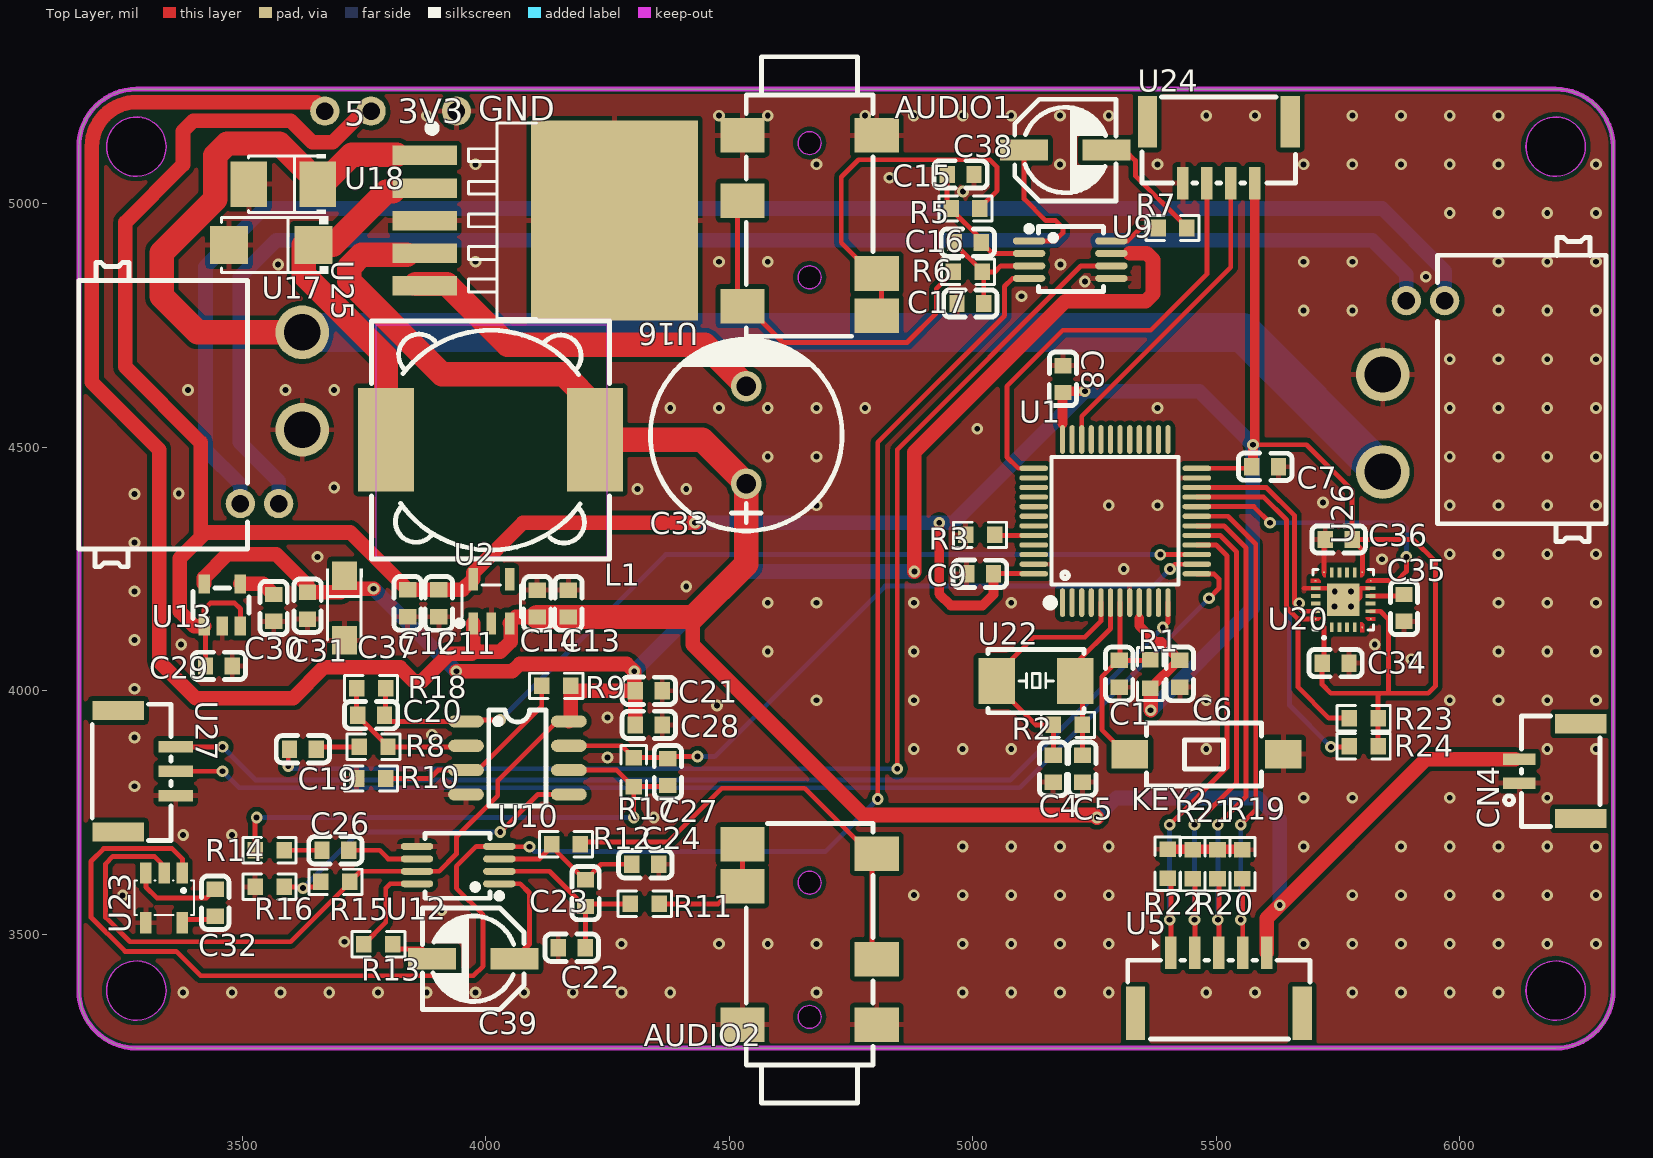
[diagram p0: Top Layer view]
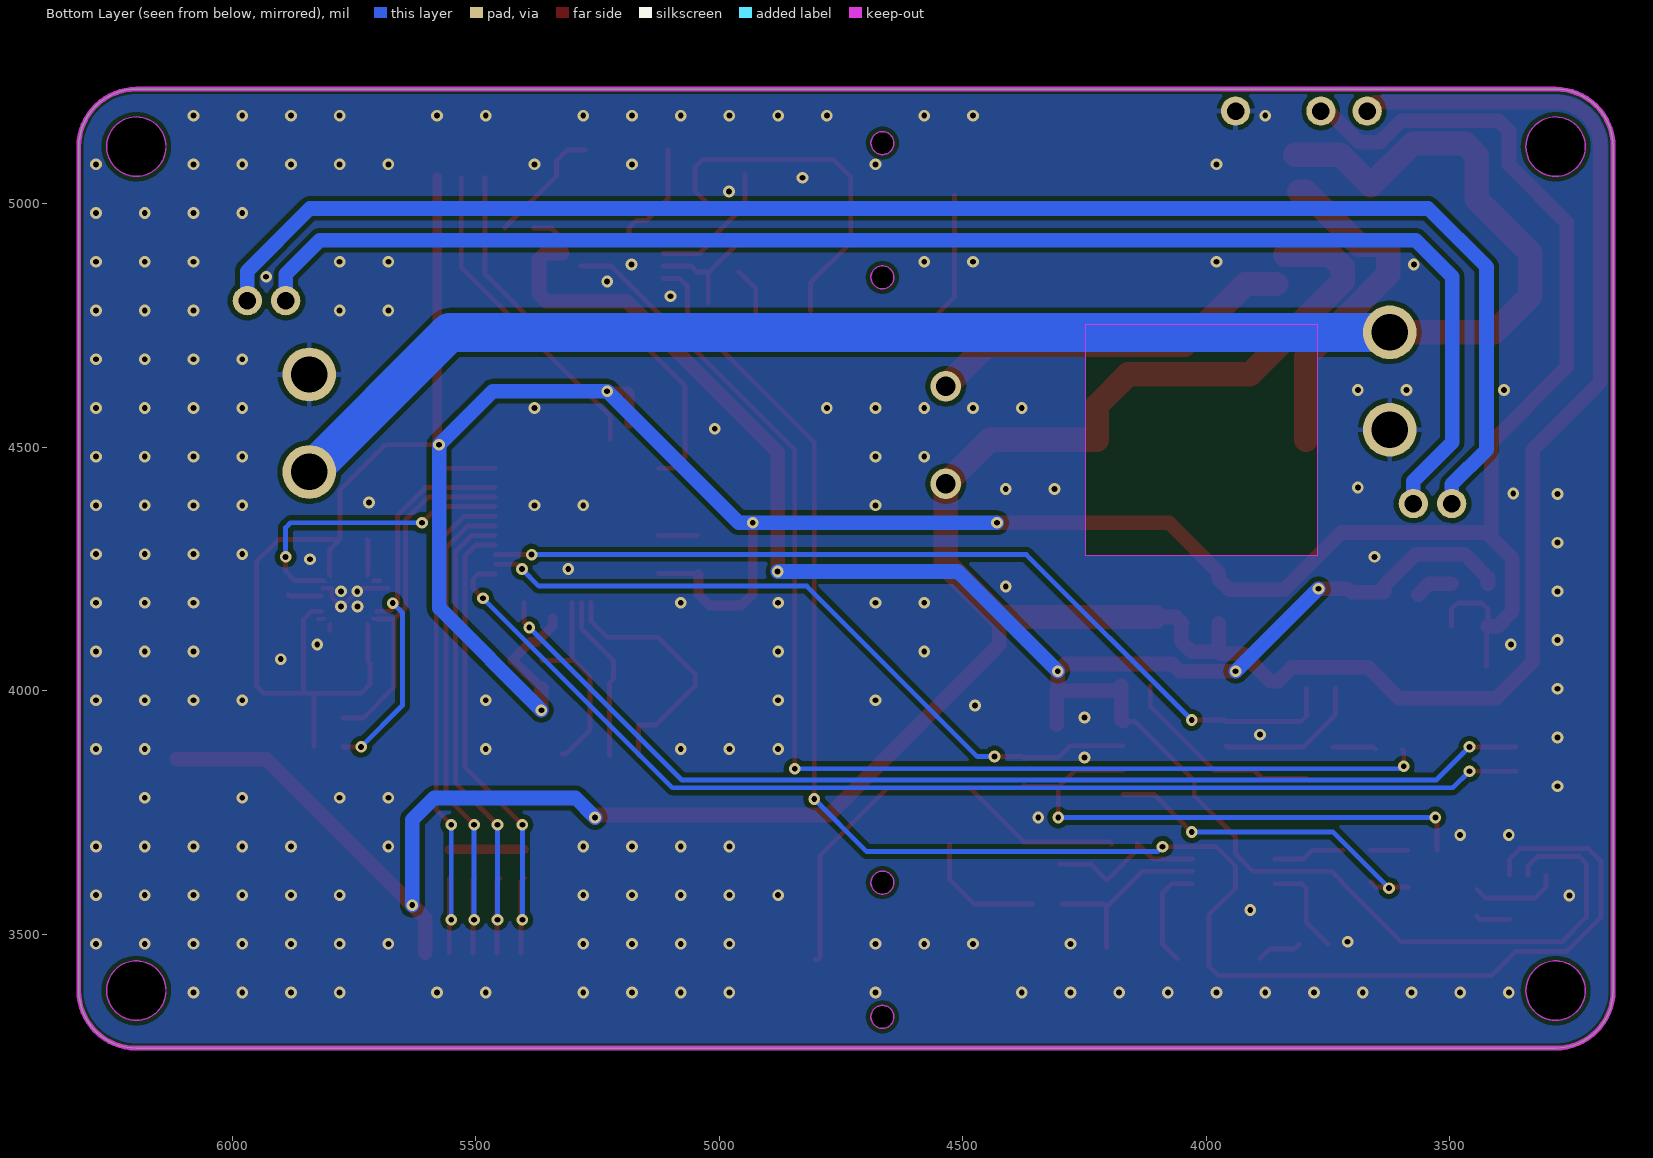
[diagram p1: Bottom Layer view, seen from below]
# Altium PCB MISC61403.pcbdoc
Units mil, origin at the board's own origin, x right, y up, seen from the top; angles counter-clockwise.
Board outline 3149.61 x 1968.5 mil, 2 copper layers (Top Layer, Bottom Layer), stack 62.206 mil thick; 79 components, 75 nets, 287 pads, 243 vias.

## Layer stack, top to bottom
Top Solder Mask Layer: solder mask 0.394, Dk 3.3
Top Layer: signal copper 1.379
Dielectric1: surface 59.449, FR4, Dk 4.5
Bottom Layer: signal copper 1.378
Bottom Solder Mask Layer: solder mask 0.394, Dk 3.3

## Board outline
3283.11,5235 ccw(c3283.11,5116.89) 3165,5116.89 3165,3384.61 ccw(c3283.11,3384.61) 3283.11,3266.5 6196.5,3266.5 ccw(c6196.5,3384.61) 6314.61,3384.61 6314.61,5116.89 ccw(c6196.5,5116.89) 6196.5,5235
cut-out: 3344.13,5116.89 cw(c3283.11,5116.89) 3222.09,5116.89 cw(c3283.11,5116.89)
cut-out: 3344.13,3384.61 cw(c3283.11,3384.61) 3222.09,3384.61 cw(c3283.11,3384.61)
cut-out: 6257.52,3384.61 cw(c6196.5,3384.61) 6135.47,3384.61 cw(c6196.5,3384.61)
cut-out: 6257.52,5116.89 cw(c6196.5,5116.89) 6135.47,5116.89 cw(c6196.5,5116.89)

## Design rules (kind name [scope] priority, off if disabled: settings)
BoardOutlineClearance Plane_innerPlane_1 [All] p2 off: genericclearance=6 ignorepadtopadclearanceinfootprint=FALSE except(0: Arc-SplitContinuation Track-SplitContinuation SMDPad-SplitContinuation THPad-SplitContinuation Via-SplitContinuation Fill-SplitContinuation Region-SplitContinuation Poly-SplitContinuation Text-SplitContinuation Hole-SplitContinuation; 6: Arc-CutoutEdge Track-CutoutEdge SMDPad-CutoutEdge THPad-CutoutEdge Via-CutoutEdge Fill-CutoutEdge Region-CutoutEdge Text-CutoutEdge Hole-CutoutEdge; 10: Poly-OutlineEdge Poly-CutoutEdge; 11.8: Arc-OutlineEdge Track-OutlineEdge SMDPad-OutlineEdge THPad-OutlineEdge Via-OutlineEdge Fill-OutlineEdge Region-OutlineEdge Text-OutlineEdge Hole-OutlineEdge)
BoardOutlineClearance Copper_copperRegion_1 [All] p4 off: genericclearance=6 ignorepadtopadclearanceinfootprint=FALSE except(0: Arc-SplitContinuation Track-SplitContinuation SMDPad-SplitContinuation THPad-SplitContinuation Via-SplitContinuation Fill-SplitContinuation Region-SplitContinuation Poly-SplitContinuation Text-SplitContinuation Hole-SplitContinuation; 6: Arc-CutoutEdge Track-CutoutEdge SMDPad-CutoutEdge THPad-CutoutEdge Via-CutoutEdge Fill-CutoutEdge Region-CutoutEdge Text-CutoutEdge Hole-CutoutEdge; 10: Poly-OutlineEdge Poly-CutoutEdge; 11.8: Arc-OutlineEdge Track-OutlineEdge SMDPad-OutlineEdge THPad-OutlineEdge Via-OutlineEdge Fill-OutlineEdge Region-OutlineEdge Text-OutlineEdge Hole-OutlineEdge)
BoardOutlineClearance safeClearance_1 [All] p6: genericclearance=6 ignorepadtopadclearanceinfootprint=FALSE except(0: Arc-SplitContinuation Track-SplitContinuation SMDPad-SplitContinuation THPad-SplitContinuation Via-SplitContinuation Fill-SplitContinuation Region-SplitContinuation Poly-SplitContinuation Text-SplitContinuation Hole-SplitContinuation; 6: Arc-CutoutEdge Track-CutoutEdge SMDPad-CutoutEdge THPad-CutoutEdge Via-CutoutEdge Fill-CutoutEdge Region-CutoutEdge Text-CutoutEdge Hole-CutoutEdge; 10: Poly-OutlineEdge Poly-CutoutEdge; 11.8: Arc-OutlineEdge Track-OutlineEdge SMDPad-OutlineEdge THPad-OutlineEdge Via-OutlineEdge Fill-OutlineEdge Region-OutlineEdge Text-OutlineEdge Hole-OutlineEdge)
Clearance Plane_innerPlane [All] p1 off: gap=6 ignorepadtopadclearanceinfootprint=FALSE except(10: Poly-Track Poly-SMDPad Poly-THPad Poly-Via Poly-Fill Poly-Region Poly-Poly Poly-Arc Poly-Text Poly-Hole)
Clearance Copper_copperRegion [All] p3 off: gap=6 ignorepadtopadclearanceinfootprint=FALSE except(10: Poly-Track Poly-SMDPad Poly-THPad Poly-Via Poly-Fill Poly-Region Poly-Poly Poly-Arc Poly-Text Poly-Hole)
Clearance safeClearance [All] p5: gap=6 ignorepadtopadclearanceinfootprint=FALSE except(10: Poly-Track Poly-SMDPad Poly-THPad Poly-Via Poly-Fill Poly-Region Poly-Poly Poly-Arc Poly-Text Poly-Hole)
DiffPairsRouting differentialPair [All] p1: maxlimit=6 minlimit=6 mostfreqgap=6 toplayer_minwidth=5 toplayer_prefwidth=10 toplayer_maxwidth=100 toplayer_mingap=6 toplayer_prefgap=6 toplayer_maxgap=6 bottomlayer_minwidth=5 bottomlayer_prefwidth=10 bottomlayer_maxwidth=100 bottomlayer_mingap=6 bottomlayer_prefgap=6 bottomlayer_maxgap=6 maxuncoupledlength=10
HoleToHoleClearance otherClearance [All] p1: gap=11.8 allowstackedmicrovias=TRUE
Length netLength [All] p1: minlimit=0 maxlimit=0
PasteMaskExpansion pasteMaskExpansion [All] p1: expansion=0
PlaneConnect innerPlane [All] p1: planeconnectstyle=Relief reliefexpansion=20 reliefentries=4 reliefconductorwidth=10 reliefairgap=10
PolygonConnect copperRegion [All] p1: connectstyle=Relief reliefconductorwidth=10 reliefentries=4 polygonreliefangle="90 Angle" airgapwidth=10 via.connectstyle=Relief via.reliefconductorwidth=10 via.reliefentries=4 via.polygonreliefangle="90 Angle" via.airgapwidth=10
RoutingVias viaSize [All] p1: holewidth=12.01 width=24.02 viastyle="Through Hole" minholewidth=11.81 minwidth=19.68 maxholewidth=236.22 maxwidth=393.7
SolderMaskExpansion solderMaskExpansion [IsVia] p1: expansion=-1000 istentingtop=TRUE
SolderMaskExpansion solderMaskExpansion [All] p2: expansion=2 istentingtop=FALSE
Width trackWidth [All] p1: maxlimit=100 minlimit=5 preferedwidth=10

## Components (designator, comment, footprint, x,y, rotation, side; value= is the part's Value field where it differs from the comment)
AUDIO1 "PJ-3420-A-SMT" AUDIO-SMD_PJ-3420-A-SMT_C319102 4665,4955 r270 top
AUDIO2 "PJ-3420-A-SMT" AUDIO-SMD_PJ-3420-A-SMT_C319102 4665,3500 r90 top
C1 "0.1u" C0603#1 5300.66,4034.95 r90 top
C4 "22pF" C0603#1 5165,3840 r90 top
C5 "22pF" C0603#1 5225,3840 r90 top
C6 "104" C0603#1 5425,4035 r90 top
C7 "104" C0603#1 5600,4460 r180 top
C8 "104" C0603#1 5185,4640 r270 top
C9 "104" C0603#1 5015,4240 r0 top
C11 "1uF" C0603#1 3904.06,4179.69 r90 top
C12 "0.1uF" C0603#1 3840,4179.69 r90 top
C13 "1uF" C0603#1 4169.81,4179.08 r270 top
C14 "0.1uF" C0603#1 4105.75,4179.08 r270 top
C15 "1nF" C0603#2 4975,5060 r0 top
C16 "1nF" C0603#2 4990,4920 r0 top
C17 "1nF" C0603#2 4995,4795 r0 top
C19 "1uF" C0603#2 3625,3880 r180 top
C20 "10nF" C0603#2 3765,3950 r180 top
C21 "100nF" C0603#2 4335,4000 r0 top
C22 "1nF" C0603#2 4176.66,3472.64 r180 top
C23 "1nF" C0603#2 4205.25,3584.83 r270 top
C24 "1nF" C0603#2 4327.81,3644.02 r180 top
C26 "1uF" C0603#2 3691.66,3672.64 r0 top
C27 "10nF" C0603#2 4374.12,3833.07 r270 top
C28 "100nF" C0603#2 4335,3930 r0 top
C29 "1uF" C0603#2 3452.51,4051.1 r0 top
C30 "470pF" C0603#2 3565,4170 r270 top
C31 "100nF" C0603#2 3634.55,4174.69 r270 top
C32 "1uF" C0603#2 3445,3565 r90 top
C33 "220uF" CAP-TH_BD10.0-P5.00-D1.0-FD 4535,4525 r90 top
C34 "10nF" C0603#2 5744.62,4056.81 r0 top
C35 "100nF" C0603#2 5885,4170 r270 top
C36 "100nF" C0603#2 5751.04,4310.62 r180 top
C37 "10uF" CAP-SMD_L3.2-W1.6-RD 3710,4170 r270 top
C38 "22uF" CAP-SMD_BD5.0-L5.3-W5.3-RD 5190,5110 r180 top
C39 "22uF" CAP-SMD_BD5.0-L5.3-W5.3-RD 3975,3450 r0 top
CN4 "GH1.25-2PWBPZ" CONN-SMD_GH1.25-2PWBPZ 6185,3835 r90 top
KEY2 "TS-1101-C-W" SW-SMD_L6.0-W3.3-LS8.0 5480,3870 r0 top
L1 "47uH" IND-SMD_L12.3-W12.3 4010,4515 r180 top
R1 "10K" R0603 5364.11,4034.42 r270 top
R2 "1M" R0603 5195,3930 r0 top
R3 "10K" R0603 5015,4320 r180 top
R5 "0" R0603 4985,4990 r180 top
R6 "0" R0603 4990,4860 r0 top
R7 "300" R0603 5410,4950 r180 top
R8 "10K" R0603 3770,3885 r0 top
R9 "10K" R0603 4145,4010 r180 top
R10 "10K" R0603 3765,3820 r0 top
R11 "0" R0603 4326.66,3562.64 r180 top
R12 "0" R0603 4165,3685 r180 top
R13 "300" R0603 3780,3480 r180 top
R14 "10K" R0603 3556.66,3672.64 r180 top
R15 "10K" R0603 3691.66,3607.64 r180 top
R16 "10K" R0603 3556.66,3597.64 r0 top
R17 "24K" R0603 4304.12,3833.07 r90 top
R18 "24K" R0603 3765,4005 r0 top
R19 "10K" R0603 5553.5,3644.17 r270 top
R20 "10K" R0603 5502.33,3644.17 r270 top
R21 "10K" R0603 5451.17,3644.17 r270 top
R22 "10K" R0603 5400,3645 r270 top
R23 "4.7K" R0603 5802.43,3944.04 r180 top
R24 "4.7K" R0603 5802.43,3886.34 r180 top
U1 "STM32F103C8T6" LQFP-48_L7.0-W7.0-P0.50-LS9.0-BL 5292.52,4348.45 r0 top
U2 "ME6211C50M5G-N" SOT-23-5_L3.0-W1.7-P0.95-LS2.8-BL 4011.77,4183.74 r0 top
U5 "BX-GH1.25-5PWT" CONN-SMD_5P-P1.25_BX-GH1.25-5PWT 5505,3400 r0 top
U9 "INA333AIDGKR" MSOP-8_L3.0-W3.0-P0.65-LS5.0-BL 5200,4885 r270 top
U10 "LMV358IDT-P" SOP-8_L4.9-W3.9-P1.27-LS6.0-BL 4065.36,3862.19 r270 top
U12 "INA333AIDGKR" MSOP-8_L3.0-W3.0-P0.65-LS5.0-BL 3943.7,3642.27 r90 top
U13 "MIC5219-3.0YM5" SOT-23-5_L2.9-W1.6-P0.95-LS2.8-BL 3459.45,4176.1 r0 top
U16 "LM2596S-5.0" TO-263-5_L10.1-W8.7-P1.70-LS14.4-BR 4070,4965 r180 top
U17 "1N5822D_SMA" SMA_L4.3-W2.6-LS5.2-RD 3560,4915 r180 top
U18 "100uF" CAP-SMD_L3.5-W2.8-FD 3585,5040 r180 top
U20 "MPU-9250" QFN-24_L3.0-W3.0-P0.40-BL-EP 5760.27,4186.81 r0 top
U22 "8MHz" OSC-SMD-2P_-L5.0-W3.2 5130,4020 r0 top
U23 "TPS60400DBVR" SOT-23-5_L3.0-W1.7-P0.95-LS2.8-BR 3340,3575 r90 top
U24 "GH1.25-4PWBPZ" CONN-SMD_GH1.25-4PWBPZ 5505,5105 r0 top
U25 "XT30PW(2+2)-M.G.B" CONN-TH_4P-XT30PW-M 3560,4560 r270 top
U26 "XT30PW(2+2)-M.G.B" CONN-TH_4P-XT30PW-M 5905,4625 r90 top
U27 "GH1.25-3PWBPZ" CONN-SMD_GH1.25-3PWBPZ 3305,3835 r270 top

## Footprints (in the part's own frame and the unit in brackets; to place one, negate y for a bottom-side part, rotate by r counter-clockwise, add the part's x,y. Pads: shape width x height; smd on the part's side, far side on the other; paste and mask are expansions set on the pad)
AUDIO-SMD_PJ-3420-A-SMT_C319102 [mm]
  rect 1.8x2.3 smd: 1(-4.7,-3.5) 2(-4.7,3.5) 3(-1.3,-3.5) 4(2.5,3.5) 5(4.7,3.5) 6(4.2,-3.5)
  Board Outline Layer circle w0.003: c2.7,0 r0.6
  Board Outline Layer circle w0.003: c-4.3,0 r0.6
  Board Outline Layer region: 2.7,0.6 2.96,0.541 3.169,0.374 3.285,0.134 3.285,-0.134 3.169,-0.374 2.96,-0.541 2.7,-0.6 2.7,-0.6 2.44,-0.541 2.231,-0.374 2.115,-0.134 2.115,0.134 2.231,0.374 2.44,0.541 2.7,0.6
  Board Outline Layer region: 2.7,0.6 2.804,0.591 2.905,0.564 3,0.52 3.086,0.46 3.16,0.386 3.22,0.3 3.264,0.205 3.291,0.104 3.3,0 3.291,-0.104 3.264,-0.205 3.22,-0.3 3.16,-0.386 3.086,-0.46 3,-0.52 2.905,-0.564 2.804,-0.591 2.7,-0.6 2.596,-0.591 2.495,-0.564 2.4,-0.52 2.314,-0.46 2.24,-0.386 2.18,-0.3 2.136,-0.205 2.109,-0.104 2.1,0 2.109,0.104 2.136,0.205 2.18,0.3 2.24,0.386 2.314,0.46 2.4,0.52 2.495,0.564 2.596,0.591
  Board Outline Layer region: -4.3,0.6 -4.04,0.541 -3.831,0.374 -3.715,0.134 -3.715,-0.134 -3.831,-0.374 -4.04,-0.541 -4.3,-0.6 -4.3,-0.6 -4.56,-0.541 -4.769,-0.374 -4.885,-0.134 -4.885,0.134 -4.769,0.374 -4.56,0.541 -4.3,0.6
  Board Outline Layer region: -4.3,0.6 -4.196,0.591 -4.095,0.564 -4,0.52 -3.914,0.46 -3.84,0.386 -3.78,0.3 -3.736,0.205 -3.709,0.104 -3.7,0 -3.709,-0.104 -3.736,-0.205 -3.78,-0.3 -3.84,-0.386 -3.914,-0.46 -4,-0.52 -4.095,-0.564 -4.196,-0.591 -4.3,-0.6 -4.404,-0.591 -4.505,-0.564 -4.6,-0.52 -4.686,-0.46 -4.76,-0.386 -4.82,-0.3 -4.864,-0.205 -4.891,-0.104 -4.9,0 -4.891,0.104 -4.864,0.205 -4.82,0.3 -4.76,0.386 -4.686,0.46 -4.6,0.52 -4.505,0.564 -4.404,0.591
  Multi-Layer board cut-out: 2.7,0.6 2.96,0.541 3.169,0.374 3.285,0.134 3.285,-0.134 3.169,-0.374 2.96,-0.541 2.7,-0.6 2.7,-0.6 2.44,-0.541 2.231,-0.374 2.115,-0.134 2.115,0.134 2.231,0.374 2.44,0.541 2.7,0.6
  Multi-Layer board cut-out: -4.3,0.6 -4.04,0.541 -3.831,0.374 -3.715,0.134 -3.715,-0.134 -3.831,-0.374 -4.04,-0.541 -4.3,-0.6 -4.3,-0.6 -4.56,-0.541 -4.769,-0.374 -4.885,-0.134 -4.885,0.134 -4.769,0.374 -4.56,0.541 -4.3,0.6
  silkscreen extent -8.8,-3.3 5.77,3.3
C0603#1 [mm]
  rect 0.8x0.9 smd paste+0 mask+0.051: 1(-0.7,0) 2(0.7,0)
  silkscreen extent -1.41,-0.71 1.39,0.72
C0603#2 [mm]
  rect 0.8x0.9 smd: 1(-0.7,0) 2(0.7,0)
  silkscreen extent -1.39,-0.71 1.39,0.71
CAP-SMD_BD5.0-L5.3-W5.3-RD [mm]
  rect 2.5x1.1 smd: 1(2.15,0) 2(-2.15,0)
  silkscreen extent -2.65,-2.65 2.64,2.65
CAP-SMD_L3.2-W1.6-RD [mm]
  rect 1.5x1.296 smd paste+0 mask+0.051: 1(-1.686,0) 2(1.686,0)
  silkscreen extent -2.06,-0.95 1.68,0.95
CAP-SMD_L3.5-W2.8-FD [mm]
  rect 1.9x2.376 smd: 1(-1.799,0) 2(1.799,0)
  silkscreen extent -2.21,-1.55 1.83,1.55
CAP-TH_BD10.0-P5.00-D1.0-FD [mm]
  round 1.6 hole 1: 1(-2.54,0) 2(2.54,0)
  silkscreen extent -5,-5 5.08,5
CONN-SMD_5P-P1.25_BX-GH1.25-5PWT [mm]
  rect 0.6x1.7 smd paste+0 mask+0.05: 1(-2.5,1.575) 2(-1.25,1.575) 3(0,1.575) 4(1.25,1.575) 5(2.5,1.575)
  rect 1x2.8 smd paste+0 mask+0.05: 6(4.35,-1.575) 7(-4.35,-1.575)
  silkscreen extent -4.75,-2.92 4.75,2.34
CONN-SMD_GH1.25-2PWBPZ [mm]
  rect 0.6x1.7 smd: 1(-0.625,1.602) 2(0.625,1.602)
  rect 1x2.7 smd: 3(2.475,-1.602) 4(-2.475,-1.598)
  silkscreen extent -2.88,-2.6 2.88,2.37
CONN-SMD_GH1.25-3PWBPZ [mm]
  rect 0.6x1.8 smd paste+0 mask+0.05: 1(-1.27,1.501) 2(0,1.501) 3(1.27,1.501)
  rect 1x2.7 smd paste+0 mask+0.05: 4(-3.164,-1.501) 5(3.164,-1.501)
  silkscreen extent -3.49,-2.85 3.62,1.25
CONN-SMD_GH1.25-4PWBPZ [mm]
  rect 0.6x1.7 smd paste+0 mask+0.05: 1(-1.875,-1.601) 2(-0.625,-1.601) 3(0.625,-1.601) 4(1.875,-1.601)
  rect 1x2.7 smd paste+0 mask+0.05: 5(-3.725,1.601) 6(3.725,1.601)
  silkscreen extent -4,-1.6 4,2.9
CONN-TH_4P-XT30PW-M [mil]
  round 110.24 hole 74.8 paste+0 mask+1.97: 1(-175.78,63.59) 2(24.22,63.59)
  round 60 hole 36 paste+0 mask+1.97: 3(175.79,15.16) 4(175.79,-63.58)
  silkscreen extent -319,-395 305,-49
IND-SMD_L12.3-W12.3 [mm]
  rect 2.9x5.4 smd: 1(-5.45,0) 2(5.45,0)
  silkscreen extent -6.2,-6.2 6.2,6.2
LQFP-48_L7.0-W7.0-P0.50-LS9.0-BL [mm]
  oval 0.27x1.5 smd paste+0 mask+0.05: 1(-2.75,-4.25) 2(-2.25,-4.25) 3(-1.75,-4.25) 4(-1.25,-4.25) 5(-0.75,-4.25) 6(-0.25,-4.25) 7(0.25,-4.25) 8(0.75,-4.25) 9(1.25,-4.25) 10(1.75,-4.25) 11(2.25,-4.25) 12(2.75,-4.25) 25(2.75,4.25) 26(2.25,4.25) 27(1.75,4.25) 28(1.25,4.25) 29(0.75,4.25) 30(0.25,4.25) 31(-0.25,4.25) 32(-0.75,4.25) 33(-1.25,4.25) 34(-1.75,4.25) 35(-2.25,4.25) 36(-2.75,4.25)
  oval 1.5x0.27 smd paste+0 mask+0.05: 13(4.25,-2.75) 14(4.25,-2.25) 15(4.25,-1.75) 16(4.25,-1.25) 17(4.25,-0.75) 18(4.25,-0.25) 19(4.25,0.25) 20(4.25,0.75) 21(4.25,1.25) 22(4.25,1.75) 23(4.25,2.25) 24(4.25,2.75) 37(-4.25,2.75) 38(-4.25,2.25) 39(-4.25,1.75) 40(-4.25,1.25) 41(-4.25,0.75) 42(-4.25,0.25) 43(-4.25,-0.25) 44(-4.25,-0.75) 45(-4.25,-1.25) 46(-4.25,-1.75) 47(-4.25,-2.25) 48(-4.25,-2.75)
  silkscreen extent -3.59,-4.46 3.3,3.34
MSOP-8_L3.0-W3.0-P0.65-LS5.0-BL [mil]
  oval 14.33x66.61 smd: 1(-38.39,-84.49) 2(-12.79,-84.49) 3(12.8,-84.49) 4(38.39,-84.49) 5(38.39,84.49) 6(12.8,84.49) 7(-12.79,84.49) 8(-38.39,84.49)
  silkscreen extent -69,-90 65,68
OSC-SMD-2P_-L5.0-W3.2 [mm]
  rect 1.9x2.4 smd paste+0 mask+0.05: 1(-2.05,0) 2(2.05,0)
  silkscreen extent -2.5,-1.65 2.5,1.65
QFN-24_L3.0-W3.0-P0.40-BL-EP [mm]
  round 0.097 smd: 1(-0.996,-1.439) 6(0.997,-1.439) 7(1.439,-0.997) 12(1.439,0.996) 13(0.997,1.439) 18(-0.997,1.439) 19(-1.439,0.997) 24(-1.439,-0.997)
  rect 0.2x0.505 smd paste-100 mask+0.051: 2(-0.6,-1.427) 3(-0.2,-1.427) 4(0.2,-1.427) 5(0.6,-1.427) 14(0.6,1.427) 15(0.2,1.427) 16(-0.2,1.427) 17(-0.6,1.427)
  rect 0.505x0.2 smd paste-100 mask+0.051: 8(1.427,-0.6) 9(1.427,-0.2) 10(1.427,0.2) 11(1.427,0.6) 20(-1.427,0.6) 21(-1.427,0.2) 22(-1.427,-0.2) 23(-1.427,-0.6)
  rect 1.7x1.7 smd paste-100 mask+0.051: 25(0,0)
  Top Layer region: -1.1,1.68 -0.9,1.68 -0.9,1.175 -1,1.174 -1.1,1.274
  Top Layer region: -1.68,-1.1 -1.274,-1.1 -1.174,-1 -1.175,-0.9 -1.68,-0.9
  Top Layer region: 1.68,-1.1 1.275,-1.1 1.175,-1 1.175,-0.9 1.68,-0.9
  Top Layer region: 1.68,1.1 1.274,1.1 1.174,1 1.175,0.9 1.68,0.9
  Top Layer region: 1.1,1.68 0.9,1.68 0.9,1.175 1,1.174 1.1,1.274
  Top Layer region: -1.1,-1.68 -0.9,-1.68 -0.9,-1.175 -1,-1.174 -1.1,-1.275
  Top Layer region: 1.1,-1.68 0.9,-1.68 0.9,-1.175 1,-1.175 1.1,-1.275
  Top Layer region: -1.68,1.1 -1.274,1.1 -1.174,1 -1.175,0.9 -1.68,0.9
  silkscreen extent -1.58,-2.05 1.58,1.58
R0603 [mil]
  rect 31.75x34.02 smd paste-3937.01 mask+2: 1(-29.66,0) 2(29.66,0)
  silkscreen extent -55,-26 55,26
SMA_L4.3-W2.6-LS5.2-RD [mm]
  rect 2x2 smd: 1(-2.2,0) 2(2.2,0)
  silkscreen extent -2.98,-1.5 2.6,1.5
SOP-8_L4.9-W3.9-P1.27-LS6.0-BL [mm]
  oval 0.63x1.865 smd: 1(-1.905,-2.682) 2(-0.635,-2.682) 3(0.635,-2.682) 4(1.905,-2.682) 5(1.905,2.682) 6(0.635,2.682) 7(-0.635,2.682) 8(-1.905,2.682)
  silkscreen extent -2.5,-1.5 2.5,1.48
SOT-23-5_L2.9-W1.6-P0.95-LS2.8-BL [mm]
  rect 0.6x1 smd paste+0 mask+0.05: 1(-0.95,-1.1) 2(0,-1.1) 3(0.95,-1.1) 4(0.95,1.1) 5(-0.95,1.1)
  silkscreen extent -1.52,-0.7 1.4,0.89
SOT-23-5_L3.0-W1.7-P0.95-LS2.8-BL [mm]
  rect 0.49x1.157 smd paste+0 mask+0.051: 1(-0.95,-1.154) 2(0,-1.154) 3(0.95,-1.154)
  rect 0.49x1.175 smd paste+0 mask+0.051: 4(0.95,1.154) 5(-0.95,1.154)
  silkscreen extent -1.8,-1.29 1.53,0.85
SOT-23-5_L3.0-W1.7-P0.95-LS2.8-BR [mm]
  rect 1.1x0.6 smd: 1(1.3,-0.95) 2(1.3,0) 3(1.3,0.95) 4(-1.3,0.95) 5(-1.3,-0.95)
  silkscreen extent -0.9,-1.55 0.9,1.55
SW-SMD_L6.0-W3.3-LS8.0 [mm]
  rect 1.9x1.5 smd paste+0 mask+0.051: 1(-4,0) 2(4,0)
  silkscreen extent -3.14,-1.67 2.86,1.63
TO-263-5_L10.1-W8.7-P1.70-LS14.4-BR [mm]
  rect 3.359x1.02 smd: 1(4.948,-3.4) 2(4.948,-1.7) 3(4.948,0) 4(4.948,1.7) 5(4.948,3.4)
  rect 8.7x10.431 smd: 6(-4.948,0)
  silkscreen extent -0.88,-5.09 4.77,5.09

## Free pads (board coordinates)
  round 60 hole 36: 1(3670,5190) 2(3765,5190) 3(3940,5190)

## Via types
v1: diameter 24.02, hole 12, Top Layer to Bottom Layer, 243 vias

## Nets (pads, with @x,y where several pads share a name; then routed paths per layer and width w, separated by ;. In a path a pad name is that pad's centre, name@x,y a point inside that pad or via, vN(x,y) a via of type N, cw(c..) or ccw(c..) an arc to the next point about the centre after c; other vN are vias at no path point)
3V: C21.1 C28.1 C31.1 C37.1 R9.1 R15.1 U9.7 U10.8 U12.7 U13.5 U23.2 | length 4477
  Top Layer w10: U23.2@3340.23,3621.38 3340.23,3639.77 3320,3660 3235,3660 3220,3645 3220,3535 3270,3485 3600,3485 3721.32,3606.32 R15.1 3743.16,3629.48 U12.7 3904.48,3629.48 3940,3665 3940,3700 4025,3785 4025,3815.53 4146.66,3937.19 U10.8
  Top Layer w30: U13.5 3422.05,4232.05 3470,4280 3570,4280 3634.55,4215.44 C31.1 3702.88,4202.25 3710,4209.37 v1(3770,4209.37) ; v1(3940,4040) 4055,4040 4070,4055 4290,4055 v1(4305,4040) 4305,4002.44 C21.1 ; U10.8 4174.66,3940.88 R9.1 4184.66,4000 C21.1 ; C28.1 C21.1 ; v1(4880,4245) 4880,4490 5190,4800 5355,4800 5370,4815 5370,4885 5357.21,4897.79 5322.4,4897.79
  Bottom Layer w30: v1(3770,4209.37) 3939.37,4040 v1(3940,4040) ; v1(4305,4040) 4510,4245 v1(4880,4245)
5V: C13.2 C14.2 C33.1 CN4.2 L1.1 pad.1 U2.1 U2.3 U5.5 U16.4 | length 6781.2
  Top Layer w30: pad.1@3660,5190 3653.2,5196.8 3653.2,5208.2 3283.11,5208.2 ccw(c3283.11,5116.89) 3259.15,5205 ccw(c3283.11,5116.89) 3201.09,5157.02 ccw(c3283.11,5116.89) 3191.8,5116.89 3191.8,4633.2 3330,4495 3330,4060 3405,3985 3605,3985 3668.01,4048.01 3824.23,4048.01 3852.24,4020 3869.09,4020 3925.09,4076 3971,4076 3980,4085 ; U2.1 3974.37,4090.63 3980,4085 ; C14.2 4062.37,4151.52 U2.3 4051.21,4136.28 4051.21,4101.21 4030,4080 3985,4080 3980,4085 ; 4425,4140 4425,4095 4775.02,3744.98 5250.02,3744.98 v1(5255,3740) ; U5.5 5603.42,3533.42 v1(5630,3560) 5929.6,3859.61 CN4.2@6112.99,3859.61
  Top Layer w50: U16.4@3838.35,4895 3745.32,4895 3720,4869.68 3720,4840.36 3910.36,4650 4160.28,4650 4224.57,4585.71 L1.1 4445,4515 C33.1 4535,4260 4426.52,4151.52 C13.2 C14.2
  Bottom Layer w30: v1(5255,3740) 5295,3780 5585,3780 5630,3735 v1(5630,3560)
24V: U16.1 U18.1 U25.1 U26.1 | length 3434.8
  Top Layer w50: U25.1 3409.21,4735.79 3335,4810 3335,4899.19 3445,5009.19 3445,5098.82 3469.67,5123.49 3576.51,5123.49 3662.5,5037.5 3725,5100 U16.1@3817.24,5100
  Bottom Layer w80: U25.1 5553.41,4735.79 U26.1@5841.41,4447.78
$1N10965: C5.2 R2.2 U1.6 U22.2 | length 344.4
  Top Layer w10: C5.2 5225,4016.65 5216.65,4025 5216.65,4061.65 5282.68,4127.68 U1.6
$1N10966: C4.2 R2.1 U1.5 U22.1 | length 532.7
  Top Layer w10: C4.2 5165.34,3867.9 R2.1 5129.45,3930 5049.29,4010.16 U22.1 5049.29,4034.14 5125.15,4110 5230,4110 5262.99,4142.99 U1.5
$1N11038: U1.35
$1N15609: C15.1 C16.2 R5.2 U9.2 | length 276.2
  Top Layer w10: C15.1 4947.44,4997.9 R5.2 4955.34,4988.87 5017.56,4926.65 C16.2 5039.77,4897.79 U9.2
$1N15623: C16.1 C17.2 R6.2 U9.3 | length 250.8
  Top Layer w10: C16.1 4962.44,4918.03 5019.66,4860.81 R6.2 ; C17.2 5022.56,4857.1 R6.2 ; U9.3 5057.74,4872.2 5045.54,4860 R6.2
$1N15783: C38.1 U9.1 | length 291.1
  Top Layer w10: C38.1 5105.35,5009.65 5150,4965 5170,4965 5185,4950 5185,4940 5168.39,4923.39 U9.1
$1N15879: C38.2 R7.1 | length 250.4
  Top Layer w10: C38.2 5312.21,5110 5333.86,5088.35 5333.86,5056.93 5439.66,4951.13 R7.1
$1N15907: R7.2 U9.8 | length 106.9
  Top Layer w10: U9.8 5317.85,4923.39 5344.46,4950 R7.2
$1N15997: C19.2 U9.6 | length 2538.8
  Top Layer w10: v1(3595,3845) 3595,3877.56 C19.2 ; v1(4845,3840) 4845,4495 5222.2,4872.2 U9.6
  Bottom Layer w10: v1(3595,3845) 3600,3840 v1(4845,3840)
$1N16023: C19.1 R8.1 | length 89.9
  Top Layer w10: C19.1 3657.56,3885 R8.1
$1N16253: C20.2 R8.2 R18.1 U10.2 | length 307.6
  Top Layer w10: R18.1 3735.34,3952.1 C20.2 3737.44,3948.35 3799.66,3886.13 R8.2 3957.56,3885 U10.2
$1N16279: R9.2 R10.2 U10.3 | length 423.7
  Top Layer w10: R10.2 3885,3820 3902.19,3837.19 U10.3 3984.06,3837.19 4115.34,3968.47 R9.2
$1N17175: C22.1 C23.2 R11.2 U12.2 | length 386
  Top Layer w10: U12.2 4131.07,3629.48 4203.28,3557.27 C23.2 ; C22.1 4205.25,3473.67 C23.2 ; R11.2 4210.62,3562.64 C23.2
$1N17182: C23.1 C24.2 R12.2 U12.3 | length 337.5
  Top Layer w10: U12.3 4110.56,3655.07 R12.2@4142,3686.51 ; R12.2@4142,3687.64 R12.2@4142,3686.51 ; C24.2 4236.88,3644.02 C23.1 4203.28,3612.39 4142,3673.67 R12.2@4142,3686.51
$1N17191: C39.1 U12.1 | length 217.2
  Top Layer w10: U12.1 4071.12,3603.88 4090,3585 4090,3480.35 C39.1
$1N17195: C39.2 R13.1 | length 93.1
  Top Layer w10: R13.1 3819.66,3470 3870.35,3470 C39.2@3890.35,3450
$1N17197: R13.2 U12.8 | length 201.4
  Top Layer w10: R13.2 3795,3524.66 3795,3595 3803.88,3603.88 U12.8
$1N17203: C26.2 U12.6 | length 147.3
  Top Layer w10: C26.2 3782.36,3672.64 3799.93,3655.07 U12.6
$1N17205: C26.1 R14.1 | length 77.8
  Top Layer w10: R14.1 C26.1
$1N17210: C27.2 R14.2 R17.1 U10.6 | length 1124.1
  Top Layer w10: R14.2 3527,3737 v1(3530,3740) ; U10.6 4269.21,3837.19 4302.99,3803.41 R17.1 ; v1(4304.12,3740) R17.1 ; C27.2 4372.02,3803.41 R17.1
  Bottom Layer w10: v1(3530,3740) v1(4304.12,3740)
$1N17215: R15.2 R16.2 U10.5 | length 705.4
  Top Layer w10: R16.2 3652,3597.64 R15.2 ; v1(4030,3710) 4107.19,3787.19 U10.5
  Bottom Layer w10: v1(3625,3595) 3740,3710 v1(4030,3710)
$1N17531: C30.1 U13.4 | length 77.2
  Top Layer w30: U13.4 3543.15,4219.41 C30.1
$1N17906: C32.1 U23.5 | length 70.1
  Top Layer w10: U23.5@3377.63,3530.83 3438.39,3530.83 C32.1
$1N17912: C32.2 U23.3 | length 182.8
  Top Layer w10: U23.3@3302.83,3621.38 3302.83,3597.17 3325,3575 3427.44,3575 C32.2
$1N18434: L1.2 U16.2 U17.1 | length 698.1
  Top Layer w50: L1.2 3795.43,4685.73 3626.61,4854.55 3626.61,4915 3686.12,4915 3796.12,5025 U16.2@3809.17,5025
$1N18564: C33.2 U16.5 | length 765.3
  Top Layer w50: U16.5@3856.73,4835 3920,4835 4045,4710 4450,4710 C33.2
$1N20884: C35.1 U20.10 | length 69.7
  Top Layer w10: U20.10 5882.12,4194.68 C35.1
-3V: U9.4 U12.4 U23.1 | length 3594.6
  Top Layer w10: U23.1@3377.63,3621.38 3377.63,3655 3356.63,3676 3216,3676 3190,3650 3190,3535 3260,3465 3365,3465 3415,3415 3975,3415 3995,3435 3995,3540 3940,3595 3940,3640 3980.66,3680.66 U12.4 4028.85,3680 v1(4090,3680) ; v1(4805,3777.98) 4805,4510 5065,4770 5065,4830 5081.61,4846.61 U9.4
  Bottom Layer w10: v1(4090,3680) 4100,3670 4697.02,3670 v1(4805,3777.98)
ADC1: C27.1 R17.2 U1.14 U10.7 | length 1465.2
  Top Layer w10: U10.7 4279.66,3887.19 R17.2 4372.02,3862.73 C27.1 4378.49,3865 v1(4435,3865) ; v1(5405,4250) 5414.87,4259.87 U1.14
  Bottom Layer w10: v1(4435,3865) 4470,3865 4820,4215 5370,4215 v1(5405,4250)
ADC2: C20.1 R18.2 U1.15 U10.1 | length 1870.3
  Top Layer w10: R18.2 3794.66,3952.1 C20.1 3805.37,3937.19 U10.1 3962.56,3940 v1(4030,3940) ; v1(5385,4279.55) U1.15
  Bottom Layer w10: v1(4030,3940) 4369.55,4279.55 v1(5385,4279.55)
ADC3: R22.2 U1.16 U5.1 | length 1022.9
  Top Layer w10: R22.2 5406.57,3608.77 U5.1 ; v1(5404.09,3725) 5521.8,3842.71 5521.8,4276.8 5499.36,4299.24 U1.16
  Bottom Layer w10: v1(5404.09,3530) v1(5404.09,3725)
ADC4: R21.2 U1.17 U5.2 | length 1040.9
  Top Layer w10: R21.2 5455.78,3609.9 U5.2 ; v1(5455.09,3725) 5541.48,3811.39 5541.48,4284.95 5507.52,4318.92 U1.17
  Bottom Layer w10: v1(5455.09,3530) v1(5455.09,3725)
ADC5: R20.2 U1.18 U5.3 | length 1061
  Top Layer w10: U1.18 5515.67,4338.61 5561.17,4293.11 5561.17,3783.2 v1(5502.97,3725) ; R20.2 5505,3611.84 U5.3
  Bottom Layer w10: v1(5502.97,3530) v1(5502.97,3725)
ADC6: R19.2 U1.19 U5.4 | length 1081.5
  Top Layer w10: U1.19 5523.82,4358.29 5580.85,4301.26 5580.85,3755.85 v1(5550,3725) ; R19.2 5554.21,3613.8 U5.4
  Bottom Layer w10: v1(5550,3530) v1(5550,3725)
BOOT0: R3.1 U1.44 | length 81
  Top Layer w10: R3.1 5045.74,4318.92 U1.44
CANH: U25.3 U26.3 | length 3009.6
  Bottom Layer w30: U25.3 3575.16,4429.85 3495,4510 3495,4850 3570,4925 5820,4925 5889.85,4855.15 U26.3@5889.85,4799.36
CANL: U25.4 U26.4 | length 3224
  Bottom Layer w30: U25.4 3496.41,4423.59 3425,4495 3425,4870 3545,4990 5840,4990 5968.59,4861.41 U26.4@5968.59,4799.36
DRY+1: AUDIO1.3 AUDIO1.6 R6.1 | length 781.2
  Top Layer w10: AUDIO1.3@4517.36,5018.11 4517.36,4807.64 4610,4715 4865,4715 4925,4775 4925,4825 4960,4860 R6.1
DRY+2: AUDIO2.3 AUDIO2.6 R12.1 | length 923.9
  Top Layer w10: R12.1 4199.66,3690 4375,3690 4485,3800 4655,3800 4792.8,3662.2 4792.8,3452.8 4796.78,3448.82 AUDIO2.3
DRY-1: AUDIO1.4 AUDIO1.5 R5.1 | length 748.9
  Top Layer w10: AUDIO1.5@4812.64,4780.43 4812.64,4837.36 4730,4920 4730,5054.65 4765.35,5090 5035,5090 5050,5075 5050,5026.47 5014.66,4991.13 R5.1
DRY-2: AUDIO2.4 AUDIO2.5 R11.1 | length 264.2
  Top Layer w10: R11.1 4477.64,3562.64 4527.2,3612.2 AUDIO2.5
GND: AUDIO1.1 AUDIO1.2 AUDIO2.1 AUDIO2.2 C1.1 C4.1 C5.1 C6.1 C7.1 C8.1 C9.1 C11.1 C12.1 C13.1 C14.1 C15.2 C17.1 C21.2 C22.2 C24.1 C28.2 C29.2 C30.2 C31.2 C34.2 C35.2 C36.2 C37.2 CN4.1 KEY2.2 pad.3 R3.2 R10.1 R16.1 R19.1 R20.1 R21.1 R22.1 U1.8 U1.23 U1.47 U2.2 U9.5 U10.4 U12.5 U13.2 U16.3 U16.6 U17.2 U18.2 U20.11 U20.18 U20.20 U20.25 U23.4 U24.1 U25.2 U26.2 U27.3 | length 398
  Top Layer w10: 5680,4210.43 U20.20 5736.65,4210.43 U20.25 5774.08,4173 v1(5776.43,4173) 5795.43,4192.01 5795.43,4210.43 U20.11@5813.65,4210.43 ; U20.18@5720.9,4243.01 5720.9,4308.04 C36.2
  Top Layer w20: R22.1 5552.67,3674.66 R19.1
  other v1: 3379.1,3380.6 3479.1,3380.6 3579.1,3380.6 3679.1,3380.6 3779.1,3380.6 3879.1,3380.6 3979.1,3380.6 4079.1,3380.6 4179.1,3380.6 4279.1,3380.6 4379.1,3380.6 4679.1,3380.6 4979.1,3380.6 5079.1,3380.6 5179.1,3380.6 5279.1,3380.6 5479.1,3380.6 5579.1,3380.6 5779.1,3380.6 5879.1,3380.6 5979.1,3380.6 6079.1,3380.6 4279.1,3480.6 4479.1,3480.6 4579.1,3480.6 4679.1,3480.6 4979.1,3480.6 5079.1,3480.6 5179.1,3480.6 5279.1,3480.6 5679.1,3480.6 5779.1,3480.6 5879.1,3480.6 5979.1,3480.6 6079.1,3480.6 6179.1,3480.6 6279.1,3480.6 3710,3485 3910,3550 3255,3580 4879.1,3580.6 4979.1,3580.6 5079.1,3580.6 5179.1,3580.6 5279.1,3580.6 5779.1,3580.6 5879.1,3580.6 5979.1,3580.6 6079.1,3580.6 6179.1,3580.6 6279.1,3580.6 4979.1,3680.6 5079.1,3680.6 5179.1,3680.6 5279.1,3680.6 5679.1,3680.6 5879.1,3680.6 5979.1,3680.6 6079.1,3680.6 6179.1,3680.6 6279.1,3680.6 3379.1,3704.1 3479.1,3704.1 4345,3740 5679.1,3780.6 5779.1,3780.6 5979.1,3780.6 6179.1,3780.6 3279.1,3804.1 4250,3863.01 4879.1,3880.6 4979.1,3880.6 5079.1,3880.6 5479.1,3880.6 6179.1,3880.6 6279.1,3880.6 3279.1,3904.1 3890,3910 4250,3945 4475,3970 4679.1,3980.6 4879.1,3980.6 5479.1,3980.6 5979.1,3980.6 6079.1,3980.6 6179.1,3980.6 6279.1,3980.6 3279.1,4004.1 5900,4065 4579.1,4080.6 4879.1,4080.6 6079.1,4080.6 6179.1,4080.6 6279.1,4080.6 3375,4095 5825,4095 3279.1,4104.1 5742.65,4173 4579.1,4180.6 4679.1,4180.6 4879.1,4180.6 5079.1,4180.6 6079.1,4180.6 6179.1,4180.6 6279.1,4180.6 3279.1,4204.1 5742.97,4204.11 5776.43,4204.11 4411.87,4214.1 5310,4250 5840,4270 3655,4275 5979.1,4280.6 6079.1,4280.6 6179.1,4280.6 6279.1,4280.6 3279.1,4304.1 4679.1,4380.6 5279.1,4380.6 5379.1,4380.6 5979.1,4380.6 6079.1,4380.6 6179.1,4380.6 6279.1,4380.6 5718.83,4386.51 3279.1,4404.1 3370,4405 4311.87,4414.1 4411.87,4414.1 3689.1,4417.5 4579.1,4480.6 4679.1,4480.6 5979.1,4480.6 6079.1,4480.6 6179.1,4480.6 6279.1,4480.6 5009.1,4538.02 4379.1,4580.6 4479.1,4580.6 4579.1,4580.6 4679.1,4580.6 4779.1,4580.6 5379.1,4580.6 5979.1,4580.6 6079.1,4580.6 6179.1,4580.6 6279.1,4580.6 3389.1,4617.5 3589.1,4617.5 3689.1,4617.5 5979.1,4680.6 6079.1,4680.6 6179.1,4680.6 6279.1,4680.6 5679.1,4780.6 5779.1,4780.6 6079.1,4780.6 6179.1,4780.6 6279.1,4780.6 5100,4810 5230,4840 5930,4850 3574.1,4874.89 5180,4875 3979.1,4880.6 4479.1,4880.6 4579.1,4880.6 5679.1,4880.6 5779.1,4880.6 6079.1,4880.6 6179.1,4880.6 6279.1,4880.6 5979.1,4980.6 6079.1,4980.6 6179.1,4980.6 6279.1,4980.6 4980,5025 4829.1,5052.96 3979.1,5080.6 4679.1,5080.6 5179.1,5080.6 5379.1,5080.6 5679.1,5080.6 5779.1,5080.6 5879.1,5080.6 5979.1,5080.6 6079.1,5080.6 6279.1,5080.6 3879.1,5180.6 4479.1,5180.6 4579.1,5180.6 4779.1,5180.6 4879.1,5180.6 4979.1,5180.6 5079.1,5180.6 5179.1,5180.6 5279.1,5180.6 5479.1,5180.6 5579.1,5180.6 5779.1,5180.6 5879.1,5180.6 5979.1,5180.6 6079.1,5180.6
IRQ0: U1.20 U20.12 | length 619.3
  Top Layer w10: U1.20 5577.02,4377.98 v1(5610,4345) ; U20.12@5816.47,4226.18 5871.18,4226.18 5890,4245 v1(5890,4275)
  Bottom Layer w10: v1(5610,4345) 5880,4345 5890,4335 v1(5890,4275)
PA0: U1.10
PA1: U1.11
PA2: U1.12 U27.1 | length 2239.3
  Top Layer w10: U27.1 v1(3460,3885) ; v1(5390,4130) 5400.79,4140.79 U1.12
  Bottom Layer w10: v1(3460,3885) 3528.01,3816.99 5076.99,3816.99 v1(5390,4130)
PA3: U1.13 U27.2 | length 2393.8
  Top Layer w10: U27.2 v1(3460,3835) ; U1.13 5460.01,4240 5495,4240 5505,4230 5505,4210 v1(5485,4190)
  Bottom Layer w10: v1(3460,3835) 3494.01,3800.99 5095.99,3800.99 v1(5485,4190)
PA8: U1.29
PA9: U1.30
PA10: U1.31
PA11: U1.32
PA12: U1.33
PA15: U1.38
PB3: U1.39
PB4: U1.40
PB5: U1.41
PB6: U1.42
PB7: U1.43
PB8: U1.45
PB9: U1.46
PB10: R23.2 U1.21 U20.24 | length 723.3
  Top Layer w10: U1.21 5597.34,4397.66 5644,4351 5644,4171 5667.81,4147.19 ; U20.24@5702.81,4147.19 5667.81,4147.19 ; R23.2 5730.96,3944.04 5667.81,4007.19 5667.81,4147.19
PB11: R24.2 U1.22 U20.23 | length 831.8
  Top Layer w10: U1.22 5602.65,4417.35 5660,4360 5660,4180 5676.81,4163.19 U20.23 ; v1(5735,3885) 5771.43,3885 R24.2
  Bottom Layer w10: v1(5670,4180) 5650,4160 5650,3970 v1(5735,3885)
PB12: U1.25
PB13: U1.26
PB14: U1.27
PB15: U1.28
PC13: U1.2
RESET: C1.2 KEY2.1 R1.1 U1.7 | length 420.1
  Top Layer w10: U1.7 5302.36,4064.2 C1.2 ; KEY2.1 5315,3870 5265,3920 5265,4028.81 5298.69,4062.51 C1.2 ; R1.1 5362.53,4062.51 C1.2
SWCLK: U1.37 U24.2 | length 914.2
  Top Layer w10: U1.37 5093.28,4456.72 5070,4480 5070,4625 5185,4740 5365,4740 5480.39,4855.39 U24.2@5480.39,5053.9
SWDAT: U1.34 U24.3 | length 664.9
  Top Layer w10: U1.34 5223.62,4563.62 5529.61,4869.61 U24.3@5529.61,5053.9
VBAT: U1.1
VCC3.3V: C6.2 C7.2 C8.2 C9.2 C11.2 C12.2 C29.1 C34.1 C36.1 pad.2 R1.2 R23.1 R24.1 U1.9 U1.24 U1.36 U1.48 U2.5 U13.1 U13.3 U20.1 U20.8 U20.13 U24.4 | length 7932.8
  Top Layer w10: U13.1 3422.05,4167.05 3435,4180 3485,4180 3496.85,4168.15 U13.3 ; C29.1 U13.1@3424.95,4129.89 ; C9.2@5042.56,4235 5048.01,4240.45 5124.93,4240.45 U1.48 ; U1.24 C7.2@5569.16,4456.72 ; v1(5575,4505) 5578.82,4505 5685,4505 5778.6,4411.4 C36.1 ; U20.1@5720.91,4130.61 5720.91,4060.66 C34.1 5717.06,4012.94 5735,3995 5836.05,3995 ; U20.13@5799.64,4243.01 5799.64,4289.58 C36.1 ; U20.8 5836.81,4163.19 5852.96,4147.04 5852.96,3995 ; R24.1 R23.1 5832.09,3991.04 5836.05,3995 ; C36.1 5904.38,4310.62 5950,4265 5950,4010 5935,3995 5852.96,3995 ; 5836.05,3995 5852.96,3995
  Top Layer w20: v1(4931.01,4345) 4931.01,4198.99 4955,4175 5020,4175 5042.56,4197.56 5042.56,4235 C9.2 ; 5184.25,4548.14 5184.25,4611.69 C8.2 5187.56,4615 v1(5230,4615) ; 5341.73,4148.73 5341.73,4133.27 5375,4100 5387.56,4100 C6.2 5421.9,4062.56 R1.2 ; C7.2 5575,4462.56 v1(5575,4505) ; v1@5578.82,4505 U24.4@5578.82,5053.9
  Top Layer w30: U13.1 3402.21,4132.79 3372.21,4162.79 3372.21,4272.21 3415.44,4315.44 ; pad.2 3750,5190 3686.21,5126.21 3643.79,5126.21 3600,5170 3400,5170 3378.79,5148.79 3378.79,5080 3260,4961.21 3260,4665 3415.44,4509.56 3415.44,4315.44 ; v1(4430,4345) 4076.73,4345 3974.37,4242.64 U2.5 3952.46,4207.25 C11.2 C12.2 3722.25,4325 3425,4325 3415.44,4315.44 ; R1.2 5365,4003.87 v1(5365,3960)
  Bottom Layer w30: v1(4430,4345) v1(4931.01,4345) 4960,4345 v1(5230,4615) 5465,4615 v1(5575,4505) 5575,4170 v1(5365,3960)
pads on no net: CN4.3 CN4.4 U1.3 U1.4 U2.4 U5.6 U5.7 U20.2 U20.3 U20.4 U20.5 U20.6 U20.7 U20.9 U20.14 U20.15 U20.16 U20.17 U20.19 U20.21 U20.22 U24.5 U24.6 U27.4 U27.5

## Polygon pours and split planes (outlines as drawn)
GND on Top Layer (solid, remove dead copper, pour order 0): 3000,5395 3000,3000 6450,3000 6450,5395
GND on Bottom Layer (solid, remove dead copper, pour order 2): 3020,5365 3020,3060 6435,3060 6435,5365

## Keep-outs
Top Layer:
  region: 3775,4750 3775,4275 4250,4275 4250,4750
Bottom Layer:
  region: 3772.5,4752.5 3772.5,4277.5 4247.5,4277.5 4247.5,4752.5
Board Outline Layer:
  region: 3344.13,5116.89 cw(c3283.11,5116.89) 3222.09,5116.89 cw(c3283.11,5116.89)
  circle w0.1: c3283.11,5116.89 r61.02
  region: 3344.13,5116.89 3343.75,5110.06 3342.6,5103.31 3340.71,5096.73 3338.09,5090.41 3334.78,5084.42 3330.82,5078.84 3326.26,5073.74 3321.16,5069.18 3315.58,5065.22 3309.59,5061.91 3303.26,5059.29 3296.69,5057.4 3289.94,5056.25 3283.11,5055.87 3276.28,5056.25 3269.53,5057.4 3262.96,5059.29 3256.63,5061.91 3250.64,5065.22 3245.06,5069.18 3239.96,5073.74 3235.4,5078.84 3231.44,5084.42 3228.13,5090.41 3225.51,5096.73 3223.62,5103.31 3222.47,5110.06 3222.09,5116.89 3222.47,5123.72 3223.62,5130.47 3225.51,5137.04 3228.13,5143.37 3231.44,5149.36 3235.4,5154.94 3239.96,5160.04 3245.06,5164.6 3250.64,5168.56 3256.63,5171.87 3262.96,5174.49 3269.53,5176.38 3276.28,5177.53 3283.11,5177.91 3289.94,5177.53 3296.69,5176.38 3303.26,5174.49 3309.59,5171.87 3315.58,5168.56 3321.16,5164.6 3326.26,5160.04 3330.82,5154.94 3334.78,5149.36 3338.09,5143.37 3340.71,5137.04 3342.6,5130.47 3343.75,5123.72
  region: 3344.13,3384.61 cw(c3283.11,3384.61) 3222.09,3384.61 cw(c3283.11,3384.61)
  circle w0.1: c3283.11,3384.61 r61.02
  region: 3344.13,3384.61 3343.75,3377.77 3342.6,3371.03 3340.71,3364.45 3338.09,3358.13 3334.78,3352.14 3330.82,3346.56 3326.26,3341.46 3321.16,3336.9 3315.58,3332.94 3309.59,3329.63 3303.26,3327.01 3296.69,3325.11 3289.94,3323.97 3283.11,3323.58 3276.28,3323.97 3269.53,3325.11 3262.96,3327.01 3256.63,3329.63 3250.64,3332.94 3245.06,3336.9 3239.96,3341.46 3235.4,3346.56 3231.44,3352.14 3228.13,3358.13 3225.51,3364.45 3223.62,3371.03 3222.47,3377.77 3222.09,3384.61 3222.47,3391.44 3223.62,3398.19 3225.51,3404.76 3228.13,3411.08 3231.44,3417.07 3235.4,3422.65 3239.96,3427.76 3245.06,3432.32 3250.64,3436.28 3256.63,3439.59 3262.96,3442.21 3269.53,3444.1 3276.28,3445.25 3283.11,3445.63 3289.94,3445.25 3296.69,3444.1 3303.26,3442.21 3309.59,3439.59 3315.58,3436.28 3321.16,3432.32 3326.26,3427.76 3330.82,3422.65 3334.78,3417.07 3338.09,3411.08 3340.71,3404.76 3342.6,3398.19 3343.75,3391.44
  region: 6257.52,3384.61 cw(c6196.5,3384.61) 6135.47,3384.61 cw(c6196.5,3384.61)
  circle w0.1: c6196.5,3384.61 r61.02
  region: 6257.52,3384.61 6257.14,3377.77 6255.99,3371.03 6254.1,3364.45 6251.48,3358.13 6248.17,3352.14 6244.21,3346.56 6239.65,3341.46 6234.54,3336.9 6228.96,3332.94 6222.97,3329.63 6216.65,3327.01 6210.08,3325.11 6203.33,3323.97 6196.5,3323.58 6189.66,3323.97 6182.92,3325.11 6176.34,3327.01 6170.02,3329.63 6164.03,3332.94 6158.45,3336.9 6153.35,3341.46 6148.79,3346.56 6144.83,3352.14 6141.52,3358.13 6138.9,3364.45 6137,3371.03 6135.86,3377.77 6135.47,3384.61 6135.86,3391.44 6137,3398.19 6138.9,3404.76 6141.52,3411.08 6144.83,3417.07 6148.79,3422.65 6153.35,3427.76 6158.45,3432.32 6164.03,3436.28 6170.02,3439.59 6176.34,3442.21 6182.92,3444.1 6189.66,3445.25 6196.5,3445.63 6203.33,3445.25 6210.08,3444.1 6216.65,3442.21 6222.97,3439.59 6228.96,3436.28 6234.54,3432.32 6239.65,3427.76 6244.21,3422.65 6248.17,3417.07 6251.48,3411.08 6254.1,3404.76 6255.99,3398.19 6257.14,3391.44
  region: 6257.52,5116.89 cw(c6196.5,5116.89) 6135.47,5116.89 cw(c6196.5,5116.89)
  circle w0.1: c6196.5,5116.89 r61.02
  region: 6257.52,5116.89 6257.14,5110.06 6255.99,5103.31 6254.1,5096.73 6251.48,5090.41 6248.17,5084.42 6244.21,5078.84 6239.65,5073.74 6234.54,5069.18 6228.96,5065.22 6222.97,5061.91 6216.65,5059.29 6210.08,5057.4 6203.33,5056.25 6196.5,5055.87 6189.66,5056.25 6182.92,5057.4 6176.34,5059.29 6170.02,5061.91 6164.03,5065.22 6158.45,5069.18 6153.35,5073.74 6148.79,5078.84 6144.83,5084.42 6141.52,5090.41 6138.9,5096.73 6137,5103.31 6135.86,5110.06 6135.47,5116.89 6135.86,5123.72 6137,5130.47 6138.9,5137.04 6141.52,5143.37 6144.83,5149.36 6148.79,5154.94 6153.35,5160.04 6158.45,5164.6 6164.03,5168.56 6170.02,5171.87 6176.34,5174.49 6182.92,5176.38 6189.66,5177.53 6196.5,5177.91 6203.33,5177.53 6210.08,5176.38 6216.65,5174.49 6222.97,5171.87 6228.96,5168.56 6234.54,5164.6 6239.65,5160.04 6244.21,5154.94 6248.17,5149.36 6251.48,5143.37 6254.1,5137.04 6255.99,5130.47 6257.14,5123.72
  lines w10: 3165,3384.61 3165,5116.89 cw(c3283.11,5116.89) 3283.11,5235 6196.5,5235 cw(c6196.5,5116.89) 6314.61,5116.89 6314.61,3384.61 cw(c6196.5,3384.61) 6196.5,3266.5 3283.11,3266.5 cw(c3283.11,3384.61) 3165,3384.61

## Silkscreen, mask and mechanical layers (free items; w line width, h text height)
Top Silkscreen Layer:
  text "GND" at 3985,5170 h50
  text "3V3" at 3820,5165 h50
  text "5" at 3710,5160 h50
Mechanical Layer:
  circle w0.1: c3283.11,5116.89 r61.02
  circle w0.1: c3283.11,3384.61 r61.02
  circle w0.1: c6196.5,3384.61 r61.02
  circle w0.1: c6196.5,5116.89 r61.02